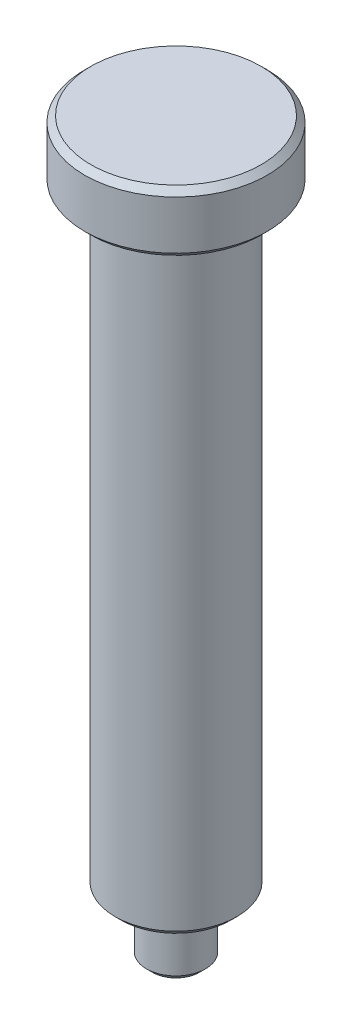
SolidWorks part; units mm, degrees
material "20#"
ref_plane "Front Plane" through (0, 0, 0) normal (0, 0, 1) x (1, 0, 0)
ref_plane "Top Plane" through (0, 0, 0) normal (0, 1, 0) x (1, 0, 0)
ref_plane "Right Plane" through (0, 0, 0) normal (1, 0, 0) x (0, 0, -1)
sketch "Sketch1" plane through (0, 0, 0) normal (1, 0, 0) x (0, 0, -1)
  line L0 (0, 0) -> (0, -60) construction
  line L1 (0, 0) -> (7.5, 0)
  line L2 (7.5, 0) -> (7.5, -5)
  line L3 (7.5, -5) -> (5, -5)
  line L4 (5, -5) -> (5, -55)
  line L5 (5, -55) -> (2.425, -55)
  line L6 (2.425, -55) -> (2.425, -60)
  line L7 (2.425, -60) -> (0, -60)
  line L8 (0, 0) -> (0, -60)
  dimension "D1" = 4.85
  dimension "D2" = 50
  dimension "D3" = 5
  dimension "D4" = 60
  dimension "D5" = 5
  dimension "D6" = 10
  dimension "D7" = 15
revolve "Revolve1" add sketch "Sketch1" angle 360 about L0
chamfer "Chamfer1" distance 0.5 angle 45 4 edges at (0, 0, 7.5) (0, -5, 7.5) (0, -55, 5) (0, -60, 2.425)
